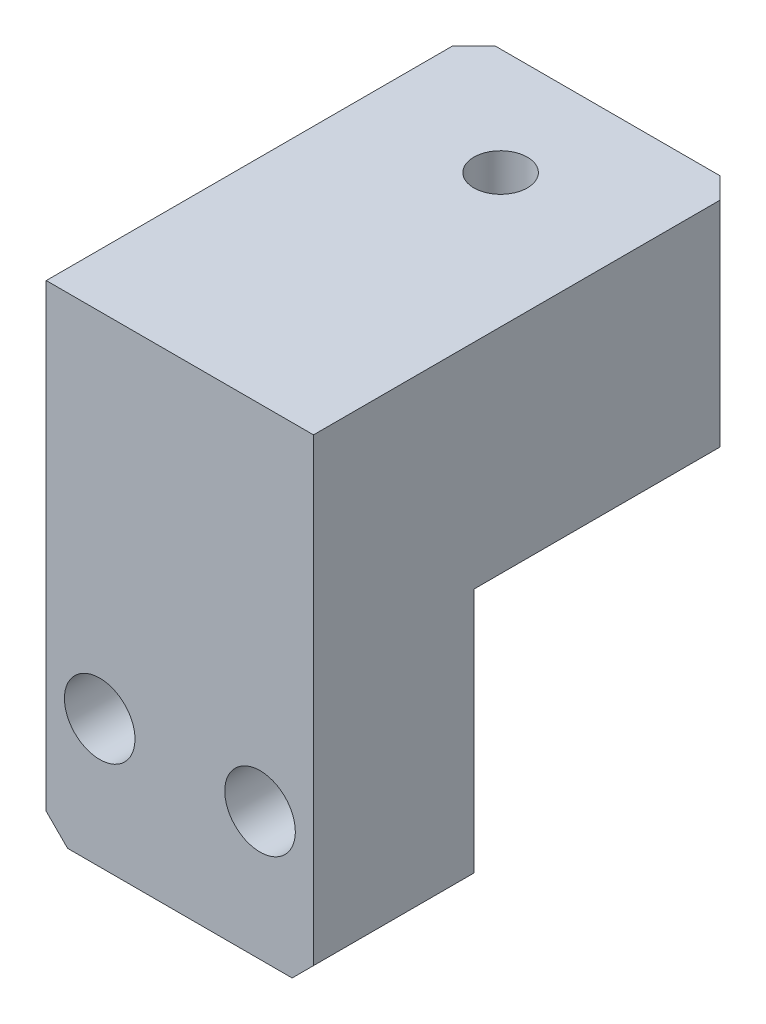
from build123d import *

# Parameters (mm, degrees)
SKETCH_1_W           = 25
SKETCH_1_H           = 40
EXTRUDE_1_DEPTH      = 20
CHAMFER_1_SIZE       = 2
HOLE_WIZARD_M6_1_D   = 5
SKETCH_6_W           = 15
SKETCH_6_H           = 25
EXTRUDE_2_DEPTH      = 25
HOLE_WIZARD_M6_1_2_D = 6.6
CHAMFER_2_SIZE       = 2


with BuildPart() as part:
    # 草图1 → 凸台-拉伸1 (new body)
    with BuildSketch(Plane(origin=(0, 0, 0), x_dir=(1, 0, 0), z_dir=(0, 1, 0))):
        with Locations((12.5, 20)):
            Rectangle(SKETCH_1_W, SKETCH_1_H)
    extrude(amount=EXTRUDE_1_DEPTH)

    # 倒角1
    chamfer_1_edges = [part.edges().sort_by_distance(p)[0] for p in [
        (0, 10, -40),
        (25, 10, -40),
    ]]
    chamfer(chamfer_1_edges, length=CHAMFER_1_SIZE)

    # Hole Wizard M6 _1 (through all)
    with Locations(Plane(origin=(0, 0, 0), x_dir=(-1, 0, 0), z_dir=(0, -1, 0))):
        with Locations((-12.5, 30)):
            Hole(HOLE_WIZARD_M6_1_D / 2)

    # 草图6 → 凸台-拉伸2 (add)
    with BuildSketch(Plane(origin=(25, 0, 0), x_dir=(0, 0, -1), z_dir=(1, 0, 0))):
        with Locations((7.5, -12.5)):
            Rectangle(SKETCH_6_W, SKETCH_6_H)
    extrude(amount=-EXTRUDE_2_DEPTH)

    # Hole Wizard M6 _1 2 (through all)
    with Locations(Plane(origin=(0, 0, -15), x_dir=(-1, 0, 0), z_dir=(0, 0, -1))):
        with Locations((-20, -13), (-5, -13)):
            Hole(HOLE_WIZARD_M6_1_2_D / 2)

    # 倒角2
    chamfer_2_edges = [part.edges().sort_by_distance(p)[0] for p in [
        (25, -25, -7.5),
        (0, -25, -7.5),
    ]]
    chamfer(chamfer_2_edges, length=CHAMFER_2_SIZE)


solid = part.part
